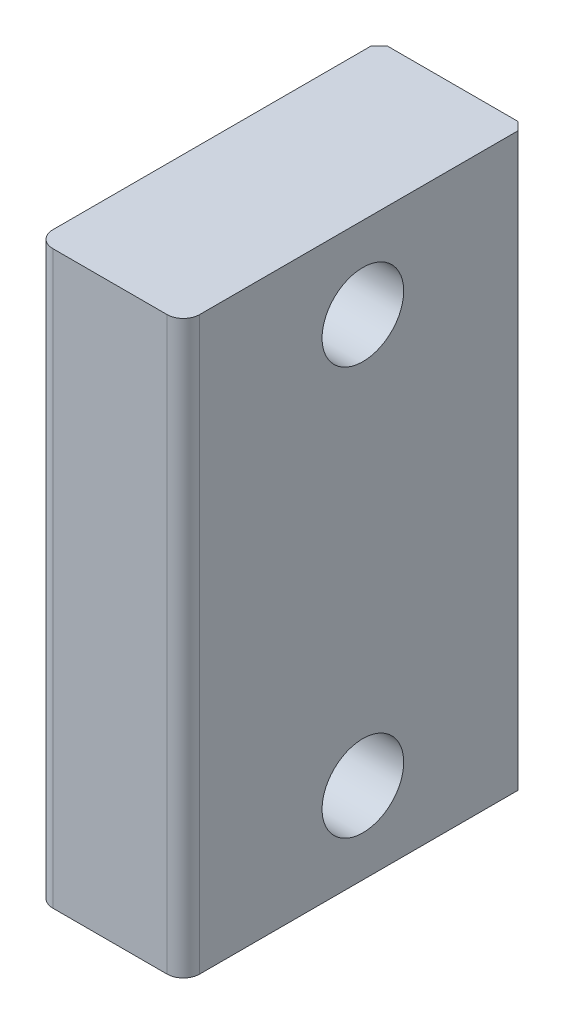
SolidWorks part; units mm, degrees
material "45"
ref_plane "Front Plane" through (0, 0, 0) normal (0, 0, 1) x (1, 0, 0)
ref_plane "Top Plane" through (0, 0, 0) normal (0, 1, 0) x (1, 0, 0)
ref_plane "Right Plane" through (0, 0, 0) normal (1, 0, 0) x (0, 0, -1)
sketch "Sketch1" plane through (0, 0, 0) normal (0, 0, 1) x (1, 0, 0)
  line L1 (0, 17.5) -> (9, 17.5)
  line L2 (0, 17.5) -> (0, -17.5)
  line L3 (0, -17.5) -> (9, -17.5)
  line L4 (9, 17.5) -> (9, -17.5)
  line L6 (-34.7216, 0) -> (46.5106, 0) construction
  dimension "D1" = 35
  dimension "D2" = 9
extrude "Boss-Extrude1" add sketch "Sketch1" along normal blind 21
hole_wizard "M6 Tapped Hole1" positions "Sketch5" profile "Sketch4" tap size "M6" standard "Gb"
sketch "Sketch5" plane through (9, 0, 0) normal (1, 0, 0) x (0, 0, -1)
  line L1 (-25.5148, 0) -> (13.5877, 0) construction
  line L4 (0, -17.5) -> (0, 17.5) construction
  point P0 (-10, 12.5)
  point P1 (-10, -12.5)
  dimension "D1" = 25
  dimension "D2" = 10
sketch "Sketch4" plane through (9, 12.5, 10) normal (0, 1, 0) x (0, 0, -1)
  line L0 (0, 0) -> (0, 16.5022)
  line L1 (0, 16.5022) -> (2.5, 15)
  line L2 (2.5, 15) -> (2.5, 0)
  line L5 (2.5, 0) -> (0, 0)
  line L10 (0, 16.5022) -> (-2.5, 15) construction
  line L11 (0, -6.35) -> (0, 107.95) construction
  dimension "螺纹孔钻头直径" = 5
  dimension "螺纹孔钻头深度" = 15
  dimension "导头角度" = 118
cosmetic thread "Hole cosmetic thread3"
cosmetic thread "Hole cosmetic thread4"
hole_wizard "M4 Tapped Hole1" positions "Sketch7" profile "Sketch6" tap size "M4" standard "Gb"
sketch "Sketch7" plane through (0, 0, 0) normal (0, 0, -1) x (-1, 0, 0)
  line L0 (-4.5, -4.5) -> (-4.5, 4.5) construction
  line L2 (-4.5, 0) -> (0, 0) construction
  line L4 (-9, -17.5) -> (-9, 17.5) construction
  point P0 (-4.5, 4.5)
  point P2 (-4.5, -4.5)
  dimension "D1" = 9
  dimension "D2" = 4.5
sketch "Sketch6" plane through (4.5, 4.5, 0) normal (1, 0, 0) x (0, 1, 0)
  line L0 (0, 0) -> (0, 15.9914)
  line L1 (0, 15.9914) -> (1.65, 15)
  line L2 (1.65, 15) -> (1.65, 0)
  line L5 (1.65, 0) -> (0, 0)
  line L10 (0, 15.9914) -> (-1.65, 15) construction
  line L11 (0, -6.35) -> (0, 107.95) construction
  dimension "螺纹孔钻头直径" = 3.3
  dimension "螺纹孔钻头深度" = 15
  dimension "导头角度" = 118
cosmetic thread "Hole cosmetic thread5"
cosmetic thread "Hole cosmetic thread6"
fillet "Fillet1" radius 1 2 edges at (0, 0, 21) (9, 0, 21)
chamfer "Chamfer1" distance 0.5 angle 45 2 edges at (0, 0, 0) (9, 0, 0)
